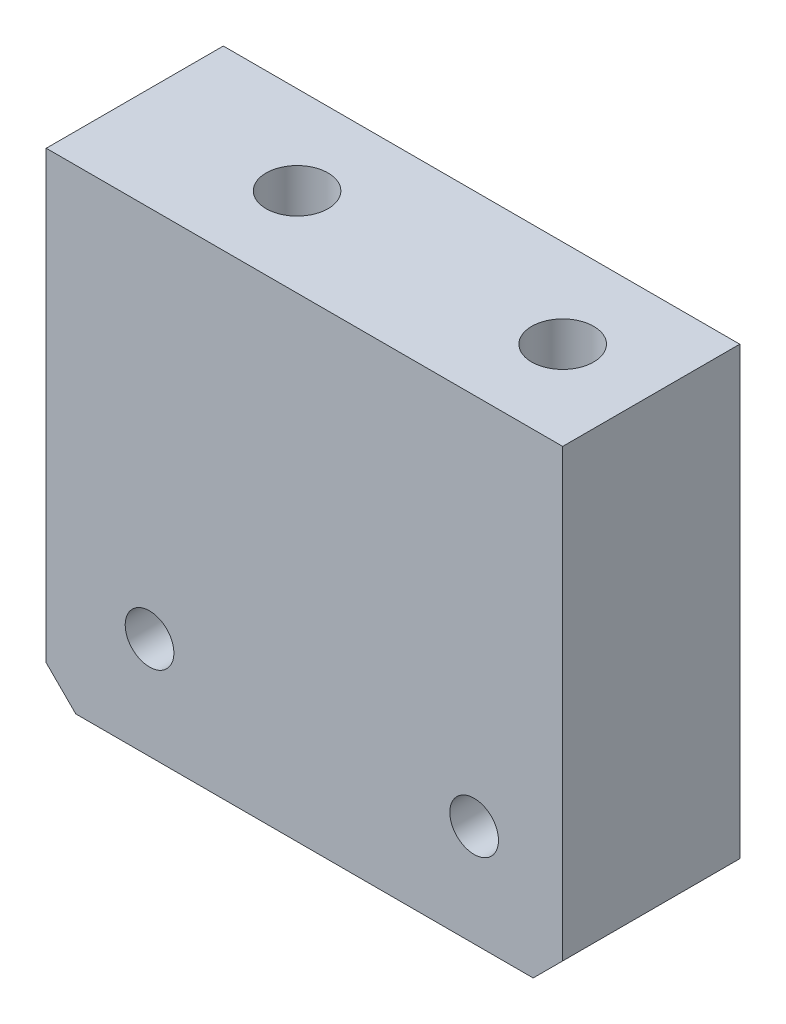
SolidWorks part; units mm, degrees
ref_plane "Front Plane" through (0, 0, 0) normal (0, 0, 1) x (1, 0, 0)
ref_plane "Top Plane" through (0, 0, 0) normal (0, 1, 0) x (1, 0, 0)
ref_plane "Right Plane" through (0, 0, 0) normal (1, 0, 0) x (0, 0, -1)
sketch "Sketch1" plane through (0, 0, 0) normal (0, 1, 0) x (1, 0, 0)
  line L1 (-17.5, 6) -> (17.5, 6)
  line L2 (-17.5, 6) -> (-17.5, -6)
  line L3 (-17.5, -6) -> (17.5, -6)
  line L4 (17.5, 6) -> (17.5, -6)
  line L5 (-17.5, 6) -> (17.5, -6) construction
  line L6 (-17.5, -6) -> (17.5, 6) construction
  point P0 (0, 0)
  dimension "D1" = 35
  dimension "D2" = 12
extrude "Boss-Extrude1" add sketch "Sketch1" along normal blind 32.2
hole_wizard "M5 Tapped Hole1" positions "3DSketch1" profile "Sketch3" tap size "M5" standard "Gb"
sketch3d "3DSketch1"
  line L0 (17.5, 32.2, 6) -> (17.5, 32.2, -6) construction
  line L1 (17.5, 32.2, -6) -> (-17.5, 32.2, -6) construction
  point P0 (11.5, 32.2, 0)
  point P2 (-6.5, 32.2, 0)
  dimension "D1" = 6
  dimension "D2" = 18
  dimension "D3" = 6
sketch "Sketch3" plane through (11.5, 32.2, 0) normal (1, 0, 0) x (0, 0, 1)
  line L0 (0, 0) -> (0, 13.6618)
  line L1 (0, 13.6618) -> (2.1, 12.4)
  line L2 (2.1, 12.4) -> (2.1, 0)
  line L5 (2.1, 0) -> (0, 0)
  line L10 (0, 13.6618) -> (-2.1, 12.4) construction
  line L11 (0, -6.35) -> (0, 107.95) construction
  dimension "螺纹孔钻头直径" = 4.2
  dimension "螺纹孔钻头深度" = 12.4
  dimension "导头角度" = 118
cosmetic thread "Cosmetic Thread1"
cosmetic thread "Cosmetic Thread2"
chamfer "Chamfer2" distance 2 angle 45 2 edges at (-17.5, 0, 0) (17.5, 0, 0)
hole_wizard "M4 Tapped Hole1" positions "3DSketch2" profile "Sketch5" tap size "M4" standard "Gb" end condition through all
sketch3d "3DSketch2"
  point P0 (11.5, 6.9, -6)
  point P2 (-10.5, 6.9, -6)
  dimension "D1" = 6
  dimension "D2" = 6.9
  dimension "D3" = 22
sketch "Sketch5" plane through (11.5, 6.9, -6) normal (1, 0, 0) x (0, 1, 0)
  line L0 (0, 0) -> (0, 12)
  line L1 (0, 12) -> (1.65, 12)
  line L2 (1.65, 12) -> (1.65, 0)
  line L5 (1.65, 0) -> (0, 0)
  line L11 (0, -6.35) -> (0, 107.95) construction
  dimension "通孔螺纹孔钻头直径" = 3.3
  dimension "通孔螺纹孔钻头深度" = 12
cosmetic thread "Cosmetic Thread3"
cosmetic thread "Cosmetic Thread4"
